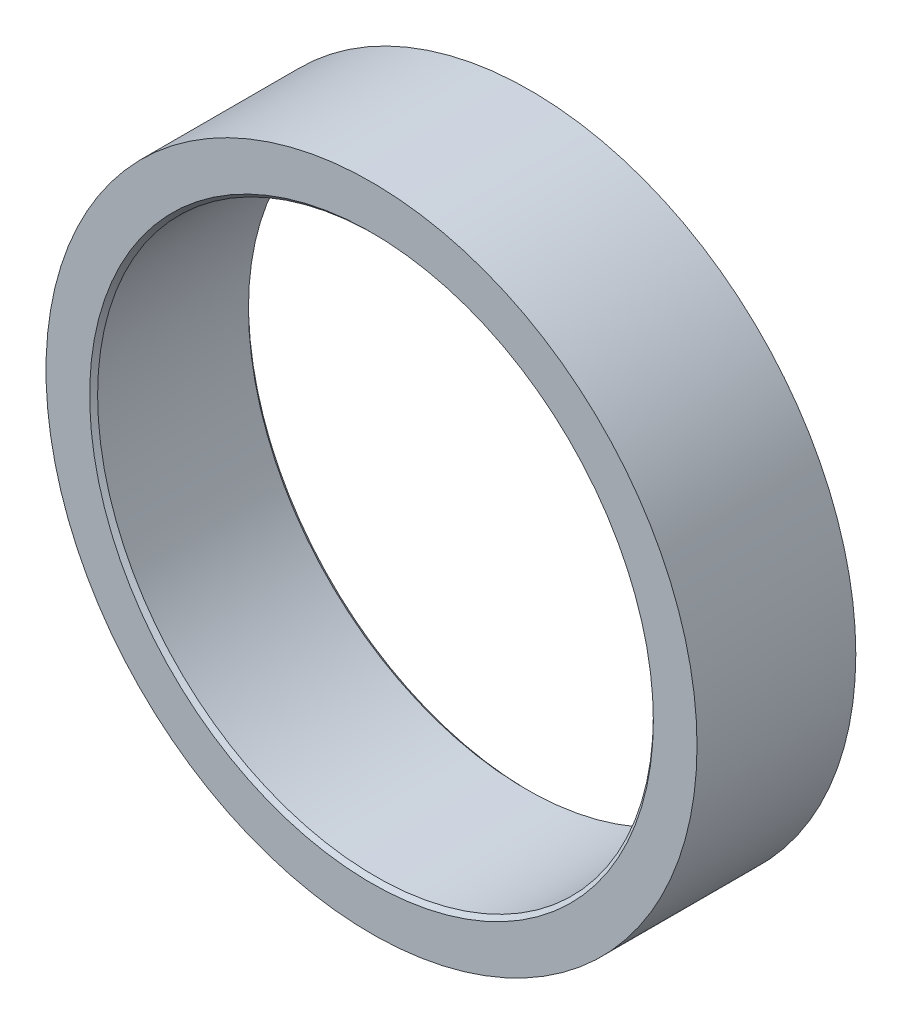
from build123d import *

# Parameters (mm, degrees)
SKETCH1_R           = 41
SKETCH1_R_2         = 35
BOSS_EXTRUDE1_DEPTH = 20
CHAMFER1_SIZE       = 0.5


with BuildPart() as part:
    # Sketch1 → Boss-Extrude1 (new body)
    with BuildSketch(Plane.XY):
        Circle(SKETCH1_R)
        Circle(SKETCH1_R_2, mode=Mode.SUBTRACT)
    extrude(amount=BOSS_EXTRUDE1_DEPTH)

    # Chamfer1
    chamfer1_edges = [part.edges().sort_by_distance(p)[0] for p in [
        (-35, 0, 0),
        (-35, 0, 20),
    ]]
    chamfer(chamfer1_edges, length=CHAMFER1_SIZE)


solid = part.part
